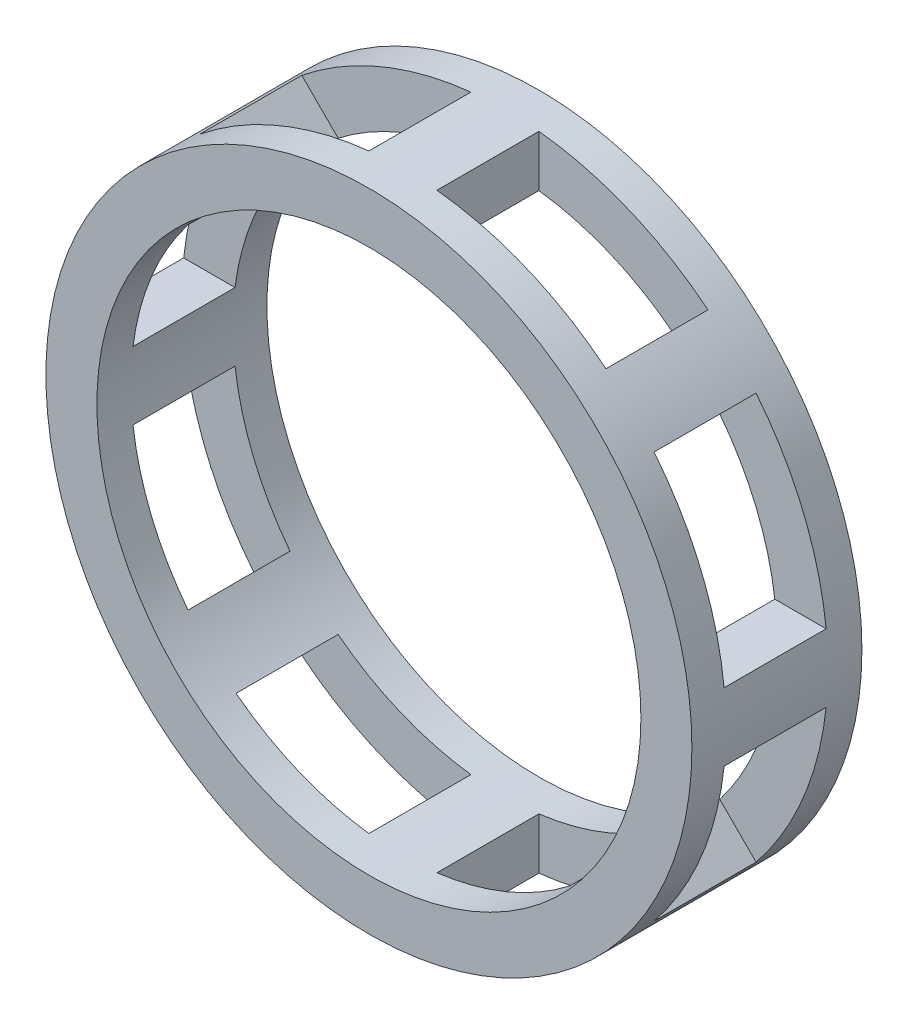
from build123d import *

# Parameters (mm, degrees)
SKETCH1_R           = 95
SKETCH1_R_2         = 80
BOSS_EXTRUDE1_DEPTH = 50
CUT_EXTRUDE1_START  = -40
SKETCH2_R           = 80
CUT_EXTRUDE1_DEPTH  = 30


with BuildPart() as part:
    # Sketch1 → Boss-Extrude1 (new body)
    with BuildSketch(Plane.XY):
        with Locations((-599.884196758, -90)):
            Circle(SKETCH1_R)
        with Locations((-599.884196758, -90)):
            Circle(SKETCH1_R_2, mode=Mode.SUBTRACT)
    extrude(amount=BOSS_EXTRUDE1_DEPTH)

    # Sketch2 → Cut-Extrude1 (cut)
    with BuildSketch(Plane.XY.offset(50).offset(CUT_EXTRUDE1_START)):
        with BuildLine():
            ThreePointArc((-679.25673609, -100), (-673.794559359, -120.614674589), (-663.080125372, -139.05379299))
            Line((-663.080125372, -139.05379299), (-624.026332382, -100))
            Line((-624.026332382, -100), (-679.25673609, -100))
        make_face()
        with BuildLine():
            ThreePointArc((-694.356414897, -100), (-687.652752347, -126.354926075), (-673.757210649, -149.730878268))
            Line((-673.757210649, -149.730878268), (-663.080125372, -139.05379299))
            ThreePointArc((-663.080125372, -139.05379299), (-673.794559359, -120.614674589), (-679.25673609, -100))
            Line((-679.25673609, -100), (-694.356414897, -100))
        make_face()
        with BuildLine():
            Line((-609.884196758, -114.142135624), (-648.937989748, -153.195928613))
            ThreePointArc((-648.937989748, -153.195928613), (-630.498871347, -163.910362601), (-609.884196758, -169.372539332))
            Line((-609.884196758, -169.372539332), (-609.884196758, -114.142135624))
        make_face()
        with BuildLine():
            Line((-648.937989748, -153.195928613), (-659.615075026, -163.873013891))
            ThreePointArc((-659.615075026, -163.873013891), (-636.239122833, -177.768555589), (-609.884196758, -184.472218138))
            Line((-609.884196758, -184.472218138), (-609.884196758, -169.372539332))
            ThreePointArc((-609.884196758, -169.372539332), (-630.498871347, -163.910362601), (-648.937989748, -153.195928613))
        make_face()
        with BuildLine():
            Line((-589.884196758, -169.372539332), (-589.884196758, -184.472218138))
            ThreePointArc((-589.884196758, -184.472218138), (-563.529270683, -177.768555589), (-540.15331849, -163.873013891))
            Line((-540.15331849, -163.873013891), (-550.830403768, -153.195928613))
            ThreePointArc((-550.830403768, -153.195928613), (-569.269522169, -163.910362601), (-589.884196758, -169.372539332))
        make_face()
        with BuildLine():
            Line((-589.884196758, -114.142135624), (-589.884196758, -169.372539332))
            ThreePointArc((-589.884196758, -169.372539332), (-569.269522169, -163.910362601), (-550.830403768, -153.195928613))
            Line((-550.830403768, -153.195928613), (-589.884196758, -114.142135624))
        make_face()
        with BuildLine():
            Line((-575.742061134, -100), (-536.688268145, -139.05379299))
            ThreePointArc((-536.688268145, -139.05379299), (-525.973834157, -120.614674589), (-520.511657426, -100))
            Line((-520.511657426, -100), (-575.742061134, -100))
        make_face()
        with BuildLine():
            Line((-536.688268145, -139.05379299), (-526.011182867, -149.730878268))
            ThreePointArc((-526.011182867, -149.730878268), (-512.115641169, -126.354926075), (-505.41197862, -100))
            Line((-505.41197862, -100), (-520.511657426, -100))
            ThreePointArc((-520.511657426, -100), (-525.973834157, -120.614674589), (-536.688268145, -139.05379299))
        make_face()
        with BuildLine():
            Line((-536.688268145, -40.94620701), (-575.742061134, -80))
            Line((-575.742061134, -80), (-520.511657426, -80))
            ThreePointArc((-520.511657426, -80), (-525.973834157, -59.385325411), (-536.688268145, -40.94620701))
        make_face()
        with BuildLine():
            Line((-520.511657426, -80), (-505.41197862, -80))
            ThreePointArc((-505.41197862, -80), (-512.115641169, -53.645073925), (-526.011182867, -30.269121732))
            Line((-526.011182867, -30.269121732), (-536.688268145, -40.94620701))
            ThreePointArc((-536.688268145, -40.94620701), (-525.973834157, -59.385325411), (-520.511657426, -80))
        make_face()
        with BuildLine():
            Line((-589.884196758, -10.627460668), (-589.884196758, -65.857864376))
            Line((-589.884196758, -65.857864376), (-550.830403768, -26.804071387))
            ThreePointArc((-550.830403768, -26.804071387), (-569.269522169, -16.089637399), (-589.884196758, -10.627460668))
        make_face()
        with BuildLine():
            ThreePointArc((-540.15331849, -16.126986109), (-563.529270683, -2.231444411), (-589.884196758, 4.472218138))
            Line((-589.884196758, 4.472218138), (-589.884196758, -10.627460668))
            ThreePointArc((-589.884196758, -10.627460668), (-569.269522169, -16.089637399), (-550.830403768, -26.804071387))
            Line((-550.830403768, -26.804071387), (-540.15331849, -16.126986109))
        make_face()
        with BuildLine():
            ThreePointArc((-609.884196758, -10.627460668), (-630.498871347, -16.089637399), (-648.937989748, -26.804071387))
            Line((-648.937989748, -26.804071387), (-609.884196758, -65.857864376))
            Line((-609.884196758, -65.857864376), (-609.884196758, -10.627460668))
        make_face()
        with BuildLine():
            ThreePointArc((-609.884196758, 4.472218138), (-636.239122833, -2.231444411), (-659.615075026, -16.126986109))
            Line((-659.615075026, -16.126986109), (-648.937989748, -26.804071387))
            ThreePointArc((-648.937989748, -26.804071387), (-630.498871347, -16.089637399), (-609.884196758, -10.627460668))
            Line((-609.884196758, -10.627460668), (-609.884196758, 4.472218138))
        make_face()
        with BuildLine():
            ThreePointArc((-673.757210649, -30.269121732), (-687.652752347, -53.645073925), (-694.356414897, -80))
            Line((-694.356414897, -80), (-679.25673609, -80))
            ThreePointArc((-679.25673609, -80), (-673.794559359, -59.385325411), (-663.080125372, -40.94620701))
            Line((-663.080125372, -40.94620701), (-673.757210649, -30.269121732))
        make_face()
        with BuildLine():
            ThreePointArc((-663.080125372, -40.94620701), (-673.794559359, -59.385325411), (-679.25673609, -80))
            Line((-679.25673609, -80), (-624.026332382, -80))
            Line((-624.026332382, -80), (-663.080125372, -40.94620701))
        make_face()
        with Locations((-599.884196758, -90)):
            Circle(SKETCH2_R)
    extrude(amount=CUT_EXTRUDE1_DEPTH, mode=Mode.SUBTRACT)


solid = part.part
